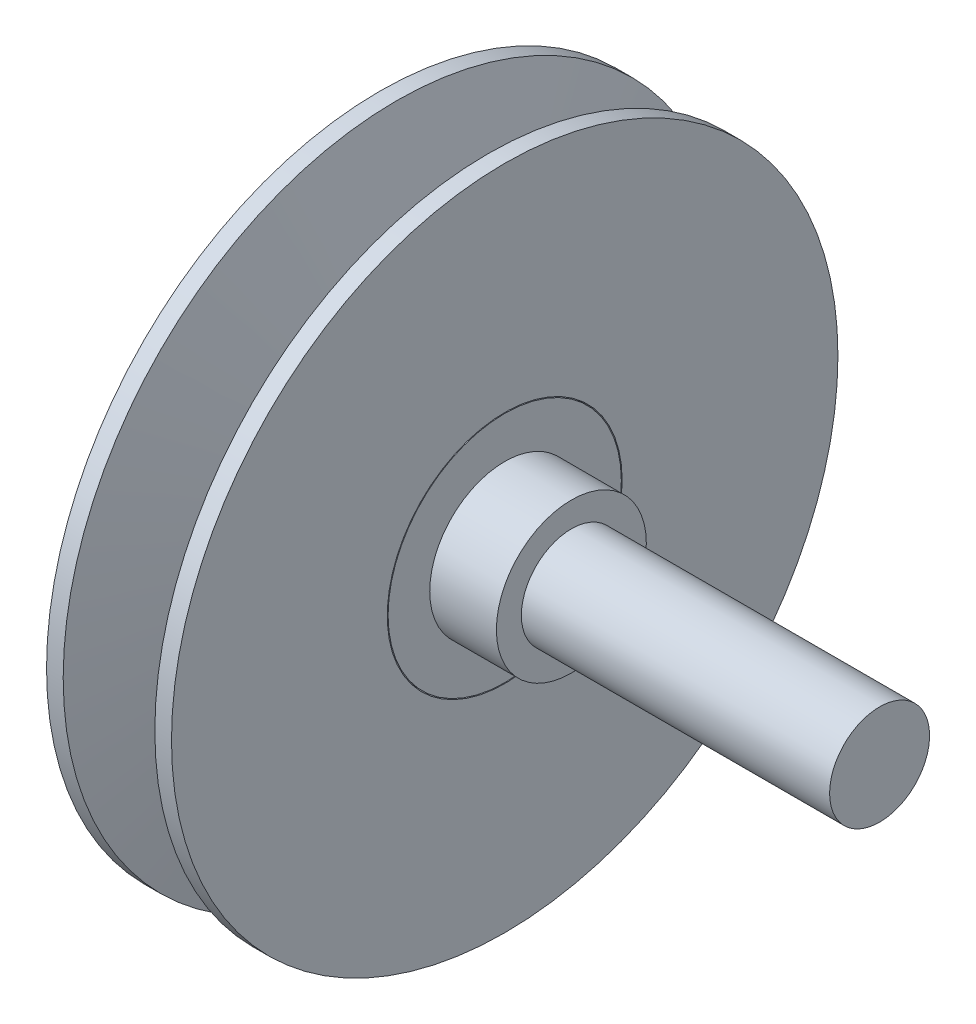
SolidWorks part; units mm, degrees
material "Q235"
ref_plane "Front" through (0, 0, 0) normal (0, 0, 1) x (1, 0, 0)
ref_plane "Top" through (0, 0, 0) normal (0, 1, 0) x (1, 0, 0)
ref_plane "Right" through (0, 0, 0) normal (1, 0, 0) x (0, 0, -1)
sketch "Sketch1" plane through (0, 0, 0) normal (0, 0, 1) x (1, 0, 0)
  line L0 (0, 0) -> (136.7778, 0) construction
  line L1 (0, 0) -> (0, 40)
  line L2 (0, 40) -> (2, 40)
  line L4 (4, 25) -> (11, 25) construction
  line L6 (13, 40) -> (15, 40)
  line L7 (15, 40) -> (15, 0)
  line L8 (15, 0) -> (0, 0)
  line L9 (2, 40) -> (13, 40) construction
  line L10 (7.5, 40) -> (7.5, 25) construction
  line L11 (2, 40) -> (5.0471, 24.5173)
  line L12 (9.9529, 24.5173) -> (13, 40)
  arc A0 (5.0471, 24.5173) -> (9.9529, 24.5173) centre (7.5, 25) ccw
  dimension "D6" = 5
  dimension "D1" = 15
  dimension "D2" = 2
  dimension "D3" = 80
  dimension "D4" = 25
revolve "Revolve1" add sketch "Sketch1" angle 360 about L0
sketch "Sketch2" plane through (0, 0, 0) normal (-1, 0, 0) x (0, 0, 1)
  circle A0 centre (0, 0) radius 6
  dimension "D1" = 12
extrude "Cut-Extrude1" cut sketch "Sketch2" against normal through all
sketch "Sketch3" plane through (0, 0, 0) normal (-1, 0, 0) x (0, 0, 1)
  circle A0 centre (0, 0) radius 14
  circle A1 centre (0, 0) radius 14.1
  dimension "D1" = 28
  dimension "D2" = 0.1
extrude "Cut-Extrude2" cut sketch "Sketch3" against normal blind 3
sketch "Sketch4" plane through (15, 0, 0) normal (1, 0, 0) x (0, 0, -1)
  circle A0 centre (0, 0) radius 14.1
  circle A1 centre (0, 0) radius 14
  circle A2 centre (0, 0) radius 14
  dimension "D1" = 0
  dimension "D2" = 0.1
extrude "Cut-Extrude3" cut sketch "Sketch4" against normal blind 3
sketch "Sketch5" plane through (15, 0, 0) normal (1, 0, 0) x (0, 0, -1)
  circle A0 centre (0, 0) radius 6
extrude "Boss-Extrude1" add sketch "Sketch5" along normal blind 45 separate body
sketch "Sketch6" plane through (15, 0, 0) normal (1, 0, 0) x (0, 0, -1)
  circle A0 centre (0, 0) radius 9
  dimension "D1" = 18
extrude "Boss-Extrude2" add sketch "Sketch6" along normal blind 8
